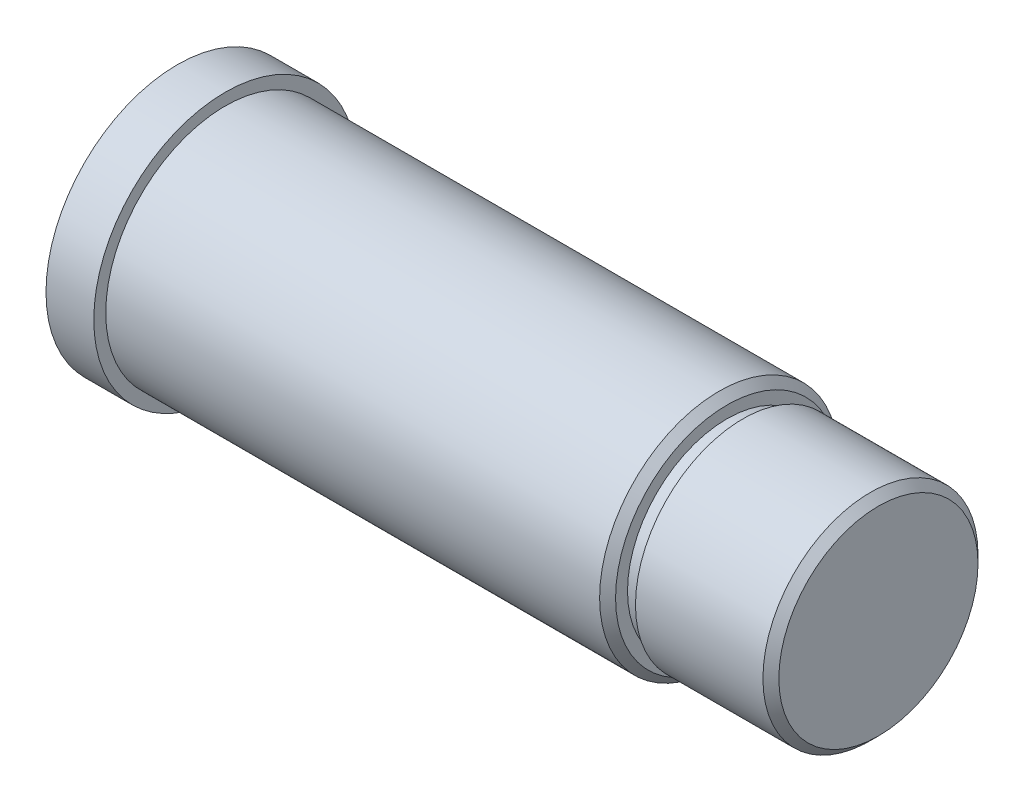
from build123d import *

# Parameters (mm, degrees)
CHAMFER_1_SIZE = 1


with BuildPart() as part:
    # 草图1 → 旋转1 (revolve)
    with BuildSketch(Plane.XY, mode=Mode.PRIVATE) as revolve_1_sk:
        Polygon((0, 0), (0, 16.5), (6, 16.5), (6, 15), (69, 15), (69, 12.5), (71, 12.5), (71, 13.5), (88, 13.5), (88, 0), align=None)
    revolve(revolve_1_sk.sketch.rotate(Axis((0, 0, 0), (1, 0, 0)), 90), axis=Axis((0, 0, 0), (1, 0, 0)))

    # 倒角1
    chamfer_1_edges = [part.edges().sort_by_distance(p)[0] for p in [
        (69, 0, -15),
        (88, 0, -13.5),
    ]]
    chamfer(chamfer_1_edges, length=CHAMFER_1_SIZE)


solid = part.part
